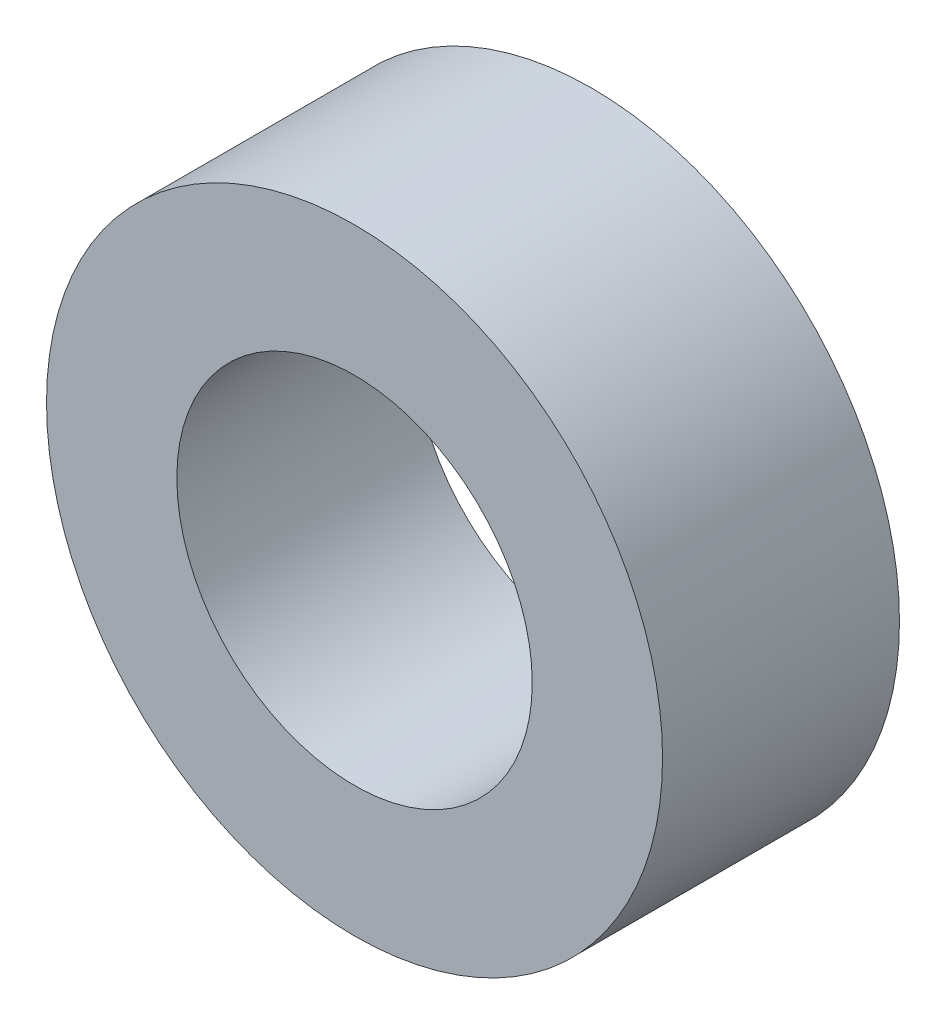
from build123d import *

# Parameters (mm, degrees)
SKETCH_1_R      = 13
SKETCH_1_R_2    = 7.5
EXTRUDE_1_DEPTH = 5


with BuildPart() as part:
    # 草图1 → 凸台-拉伸1 (new, symmetric)
    with BuildSketch(Plane.XY):
        Circle(SKETCH_1_R)
        Circle(SKETCH_1_R_2, mode=Mode.SUBTRACT)
    extrude(amount=EXTRUDE_1_DEPTH, both=True)


solid = part.part
